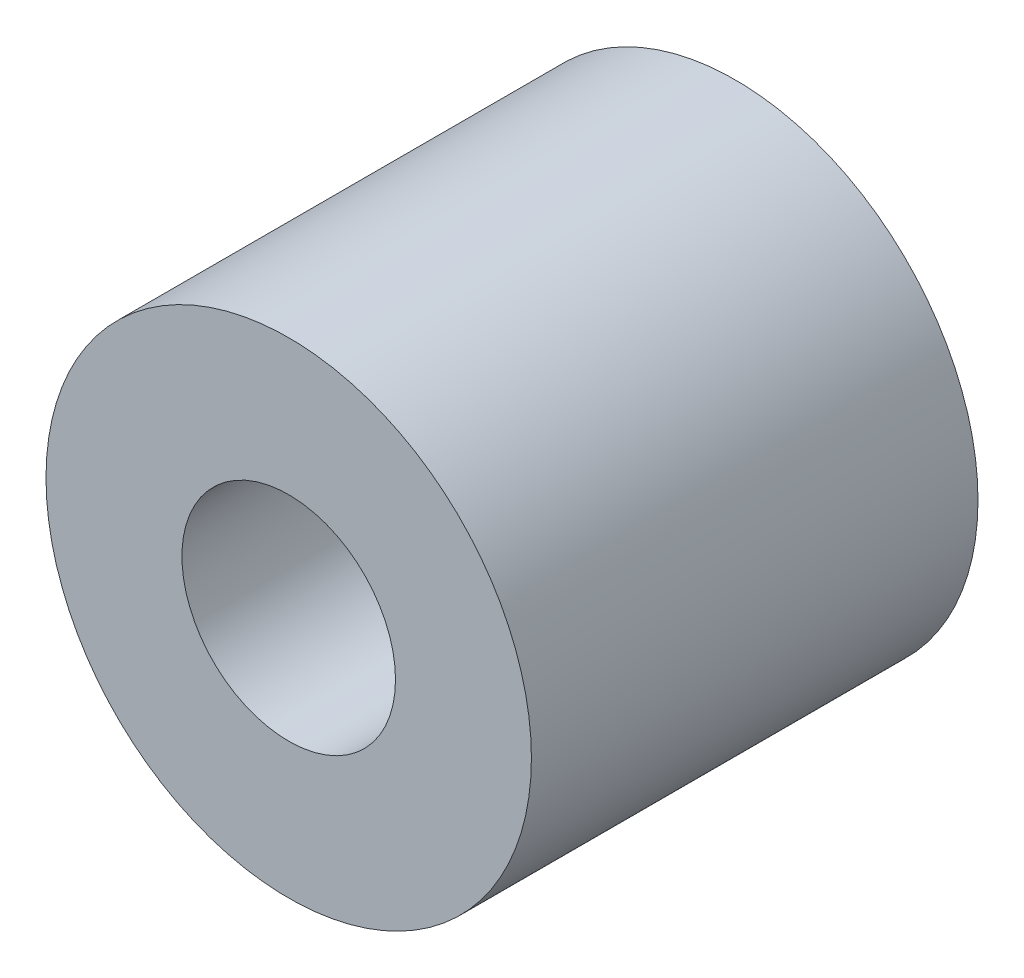
from build123d import *

# Parameters (mm, degrees)
SKETCH_1_R                   = 12.5
EXTRUDE_1_DEPTH              = 23
HOLE_WIZARD_M6_1_D           = 6.6
HOLE_WIZARD_M6_1_CBORE_D     = 11
HOLE_WIZARD_M6_1_CBORE_DEPTH = 16.8


with BuildPart() as part:
    # 草图1 → 凸台-拉伸1 (new body)
    with BuildSketch(Plane.XY):
        Circle(SKETCH_1_R)
    extrude(amount=EXTRUDE_1_DEPTH)

    # M6 六角圆柱头螺钉的柱形沉头孔1 (through all)
    with Locations(Plane.XY.offset(23)):
        with Locations((0, 0)):
            CounterBoreHole(HOLE_WIZARD_M6_1_D / 2, HOLE_WIZARD_M6_1_CBORE_D / 2, HOLE_WIZARD_M6_1_CBORE_DEPTH)


solid = part.part
